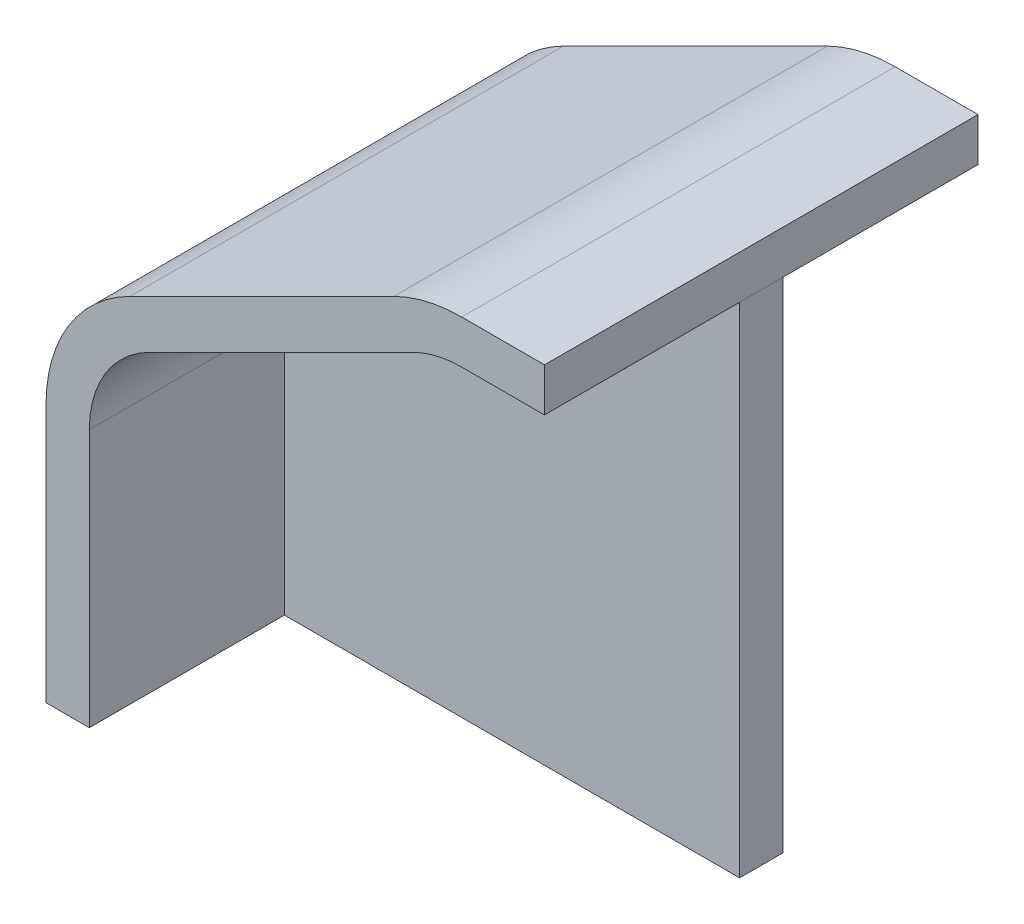
SolidWorks part; units mm, degrees
material "Q345"
ref_plane "前视基准面" through (0, 0, 0) normal (0, 0, 1) x (1, 0, 0)
ref_plane "上视基准面" through (0, 0, 0) normal (0, 1, 0) x (1, 0, 0)
ref_plane "右视基准面" through (0, 0, 0) normal (1, 0, 0) x (0, 0, -1)
sketch "草图1" plane through (0, 0, 0) normal (0, 0, 1) x (1, 0, 0)
  line L0 (0, 0) -> (210, 0)
  line L1 (0, 0) -> (0, 119.0983)
  line L2 (171.8034, 230) -> (210, 230)
  line L3 (210, 230) -> (210, 0)
  line L4 (149.4427, 224.7214) -> (27.6393, 163.8197)
  arc A0 (149.4427, 224.7214) -> (171.8034, 230) centre (171.8034, 180) cw
  arc A1 (0, 119.0983) -> (27.6393, 163.8197) centre (50, 119.0983) cw
  point P8 (160, 230)
  point P11 (0, 150)
  dimension "D5" = 50
  dimension "D6" = 50
  dimension "D1" = 150
  dimension "D2" = 210
  dimension "D3" = 230
  dimension "D4" = 50
extrude "凸台-拉伸1" add sketch "草图1" along normal blind 20
ref_plane "基准面1" through (0, 0, 10) normal (0, 0, 1) x (1, 0, 0)
sketch "草图2" plane through (0, 0, 10) normal (0, 0, 1) x (1, 0, 0)
  line L0 (210, 250) -> (171.8034, 250)
  line L1 (140.4984, 242.6099) -> (18.695, 181.7082)
  line L2 (-20, 119.0983) -> (-20, 0)
  line L3 (0, 0) -> (-20, 0)
  line L4 (210, 250) -> (210, 230)
  line L5 (0, 119.0983) -> (0, 0)
  line L6 (0, 0) -> (210, 0)
  line L7 (210, 0) -> (210, 230)
  line L8 (210, 230) -> (171.8034, 230)
  line L9 (149.4427, 224.7214) -> (27.6393, 163.8197)
  line L10 (0, 119.0983) -> (0, 0)
  line L13 (210, 230) -> (171.8034, 230)
  line L14 (149.4427, 224.7214) -> (27.6393, 163.8197)
  arc A0 (171.8034, 250) -> (140.4984, 242.6099) centre (171.8034, 180) ccw
  arc A1 (18.695, 181.7082) -> (-20, 119.0983) centre (50, 119.0983) ccw
  arc A2 (171.8034, 230) -> (149.4427, 224.7214) centre (171.8034, 180) ccw
  arc A3 (27.6393, 163.8197) -> (0, 119.0983) centre (50, 119.0983) ccw
  arc A4 (171.8034, 230) -> (149.4427, 224.7214) centre (171.8034, 180) ccw
  arc A5 (27.6393, 163.8197) -> (0, 119.0983) centre (50, 119.0983) ccw
  dimension "D1" = 0
  dimension "D2" = 20
extrude "凸台-拉伸2" add sketch "草图2" along normal mid plane 200 separate body
